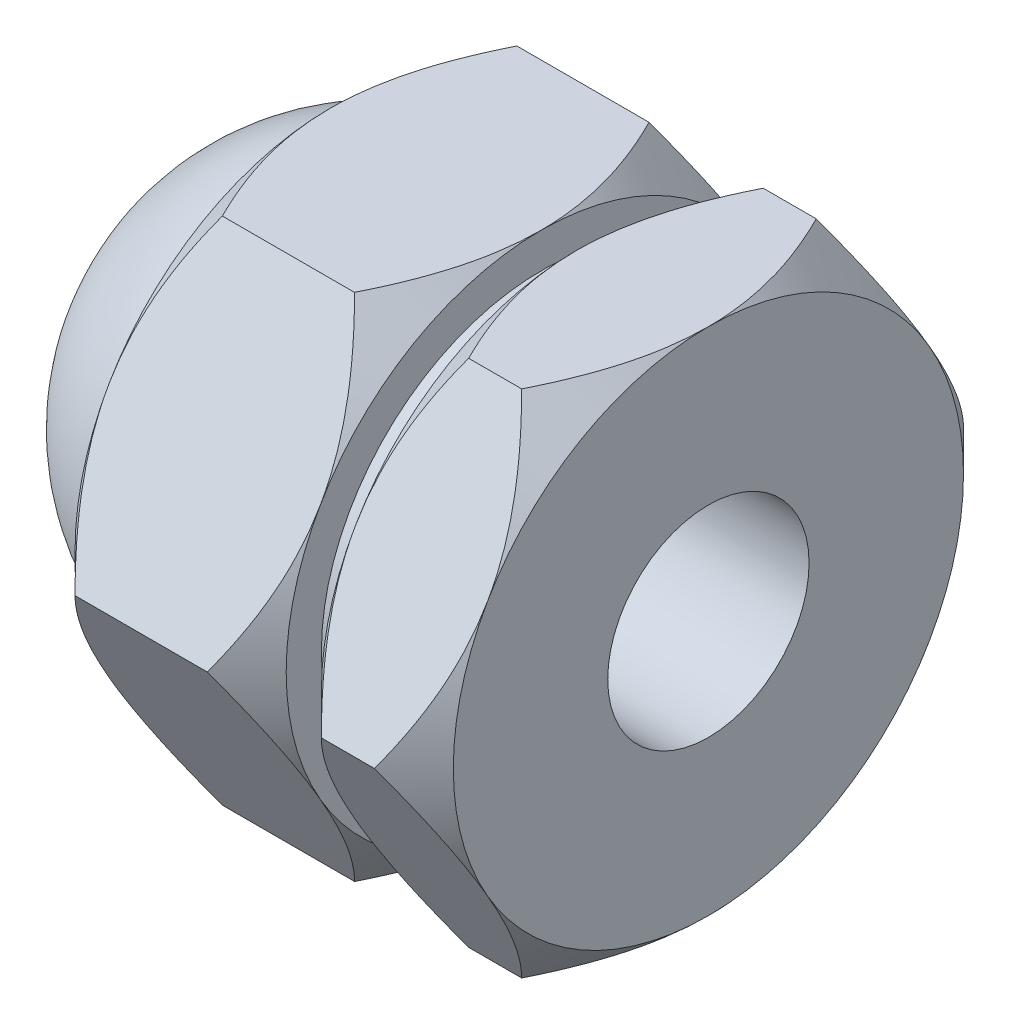
SolidWorks part; units mm, degrees
ref_plane "Front Plane" through (0, 0, 0) normal (0, 0, 1) x (1, 0, 0)
ref_plane "Top Plane" through (0, 0, 0) normal (0, 1, 0) x (1, 0, 0)
ref_plane "Right Plane" through (0, 0, 0) normal (1, 0, 0) x (0, 0, -1)
sketch "Sketch1" plane through (0, 0, 0) normal (0, 0, 1) x (1, 0, 0)
  line L0 (0, 0) -> (50000, 0) construction
  line L1 (0, 5.7225) -> (0, 7.2225)
  line L4 (8.5, 13) -> (8.5, 14.5)
  line L5 (8.5, 14.5) -> (20.5, 14.5)
  line L6 (20.5, 14.5) -> (20.5, 12.5)
  line L7 (20.5, 12.5) -> (22.5, 12.5)
  line L9 (30, 14.5) -> (30, 0)
  line L10 (15, 5.7225) -> (0, 5.7225)
  line L11 (15, 5.7225) -> (15, 0)
  line L12 (30, 0) -> (15, 0)
  line L13 (22.5, 12.5) -> (22.5, 14.5)
  line L14 (22.5, 14.5) -> (30, 14.5)
  arc A0 (8.5, 13) -> (0, 7.2225) centre (11.1227, 0) ccw
  dimension "D2" = 1.5
  dimension "D3" = 1.5
  dimension "D4" = 2
  dimension "D5" = 12
  dimension "D6" = 7.5
  dimension "D7" = 29
  dimension "D8" = 30
  dimension "D9" = 11.445
  dimension "D10" = 2
  dimension "D11" = 15
revolve "Revolve1" add sketch "Sketch1" angle 360 about L0
cosmetic thread "Cosmetic Thread1"
cosmetic thread "Cosmetic Thread2"
sketch "Sketch2" plane through (20.5, 0, 0) normal (1, 0, 0) x (0, 0, -1)
  line L1 (16.7432, 0) -> (8.3716, 14.5)
  line L2 (8.3716, 14.5) -> (-8.3716, 14.5)
  line L3 (-8.3716, 14.5) -> (-16.7432, 0)
  line L4 (-16.7432, 0) -> (-8.3716, -14.5)
  line L5 (-8.3716, -14.5) -> (8.3716, -14.5)
  line L6 (8.3716, -14.5) -> (16.7432, 0)
  circle A0 centre (0, 0) radius 14.5 construction
  circle A1 centre (0, 0) radius 14.5 construction
  circle A2 centre (0, 0) radius 12.5
  dimension "D1" = 2
extrude "Boss-Extrude1" add sketch "Sketch2" against normal up to surface (12 mm away) up to face at (8.5, 0, 13)
sketch "Sketch6" plane through (30, 0, 0) normal (1, 0, 0) x (0, 0, -1)
  line L1 (16.7432, 0) -> (8.3716, 14.5)
  line L2 (8.3716, 14.5) -> (-8.3716, 14.5)
  line L3 (-8.3716, 14.5) -> (-16.7432, 0)
  line L4 (-16.7432, 0) -> (-8.3716, -14.5)
  line L5 (-8.3716, -14.5) -> (8.3716, -14.5)
  line L6 (8.3716, -14.5) -> (16.7432, 0)
  circle A0 centre (0, 0) radius 14.5 construction
  circle A1 centre (0, 0) radius 14.5 construction
  circle A2 centre (0, 0) radius 12.5
  dimension "D1" = 2
extrude "Boss-Extrude2" add sketch "Sketch6" against normal up to surface (7.5 mm away) up to face at (22.5, 0, 12.5)
sketch "Sketch3" plane through (0, 0, 0) normal (0, 1, 0) x (1, 0, 0)
  line L0 (0, 0) -> (-50000, 0) construction
  line L2 (18.2568, 16.7432) -> (20.5, 14.5)
  line L3 (8.5, 16.7432) -> (20.5, 16.7432) construction
  line L4 (20.5, 16.7432) -> (20.5, 8.3716) construction
  line L5 (20.5, 14.5) -> (20.5, 16.7432)
  line L6 (20.5, 16.7432) -> (18.2568, 16.7432)
  line L7 (24.7432, 16.7432) -> (22.5, 14.5)
  line L8 (8.5, 14.5) -> (10.7432, 16.7432)
  line L9 (8.5, 8.3716) -> (8.5, 16.7432) construction
  line L10 (10.7432, 16.7432) -> (8.5, 16.7432)
  line L11 (8.5, 16.7432) -> (8.5, 14.5)
  line L12 (22.5, 16.7432) -> (30, 16.7432) construction
  line L13 (22.5, 8.3716) -> (22.5, 16.7432) construction
  line L14 (22.5, 14.5) -> (22.5, 16.7432)
  line L15 (22.5, 16.7432) -> (24.7432, 16.7432)
  line L16 (27.7568, 16.7432) -> (30, 16.7432)
  line L17 (30, 16.7432) -> (30, 14.5)
  line L18 (30, 16.7432) -> (30, 8.3716) construction
  line L19 (30, 14.5) -> (27.7568, 16.7432)
  dimension "D1" = 45
  dimension "D2" = 29
  dimension "D3" = 45
  dimension "D4" = 45
revolve "Cut-Revolve1" cut sketch "Sketch3" angle 360 about L0
sketch "Sketch5" plane through (15, 0, 0) normal (-1, 0, 0) x (0, 0, 1)
  circle A0 centre (0, 0) radius 1
  dimension "D1" = 2
extrude "Cut-Extrude2" cut sketch "Sketch5" against normal through all
sketch "Sketch7" plane through (30, 0, 0) normal (1, 0, 0) x (0, 0, -1)
  circle A0 centre (0, 0) radius 5.7225
  dimension "D1" = 11.445
extrude "Cut-Extrude3" cut sketch "Sketch7" against normal up to surface (15 mm away) up to face at (15, 0, 1)
